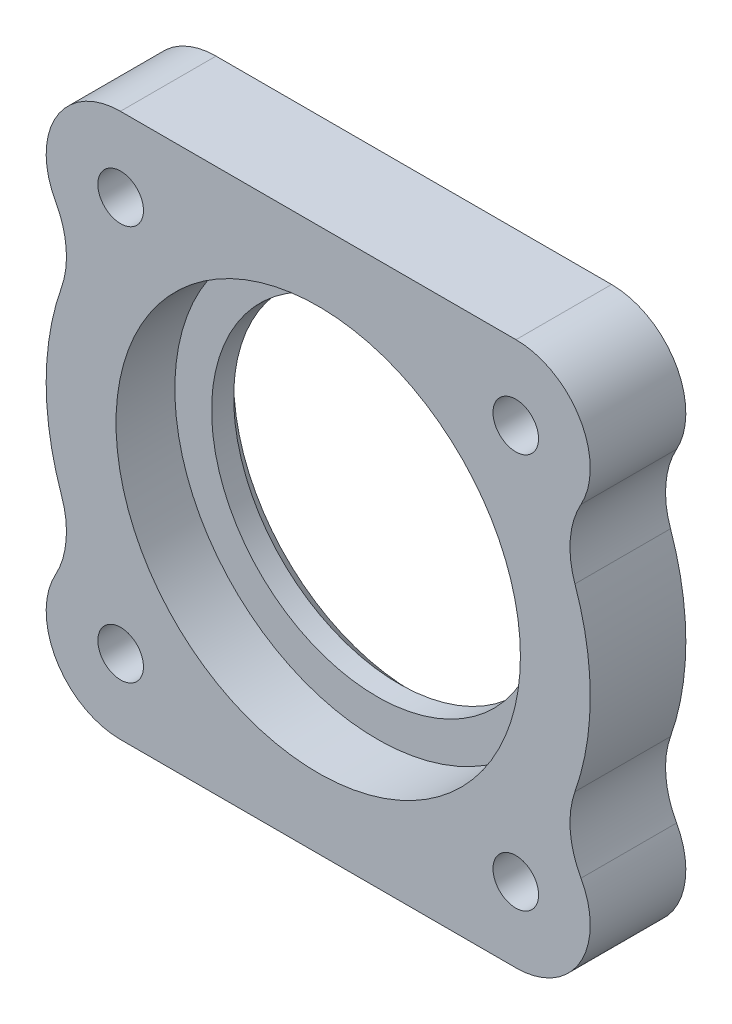
from build123d import *

# Parameters (mm, degrees)
EXTRUDE_1_DEPTH         = 13
HOLE_WIZARD_6_2_6_2_1_D = 6.2
SKETCH_4_R              = 27.5
CUT_EXTRUDE_1_DEPTH     = 8
CUT_EXTRUDE_2_REACH     = 54.934
SKETCH_5_R              = 22.5
CHAMFER_1_SIZE          = 2


with BuildPart() as part:
    # 草图1 → 凸台-拉伸1 (new body)
    with BuildSketch(Plane.XY):
        with BuildLine():
            Line((37, 0), (-37, 0))
            ThreePointArc((-37, 0), (-36.475571993, -6.2074671), (-34.917154173, -12.238968276))
            ThreePointArc((-34.917154173, -12.238968276), (-34.283867545, -17.214225736), (-35.739390486, -22.013776935))
            ThreePointArc((-35.739390486, -22.013776935), (-35.59944978, -32.031235087), (-26.9, -37))
            Line((-26.9, -37), (26.9, -37))
            ThreePointArc((26.9, -37), (35.59944978, -32.031235087), (35.739390486, -22.013776935))
            ThreePointArc((35.739390486, -22.013776935), (34.283867545, -17.214225736), (34.917154173, -12.238968276))
            ThreePointArc((34.917154173, -12.238968276), (36.475571993, -6.2074671), (37, 0))
        make_face()
        with BuildLine():
            Line((26.9, 37), (-26.9, 37))
            ThreePointArc((-26.9, 37), (-35.59944978, 32.031235087), (-35.739390486, 22.013776935))
            ThreePointArc((-35.739390486, 22.013776935), (-34.283867545, 17.214225736), (-34.917154173, 12.238968276))
            ThreePointArc((-34.917154173, 12.238968276), (-36.475571993, 6.2074671), (-37, 0))
            Line((-37, 0), (37, 0))
            ThreePointArc((37, 0), (36.475571993, 6.2074671), (34.917154173, 12.238968276))
            ThreePointArc((34.917154173, 12.238968276), (34.283867545, 17.214225736), (35.739390486, 22.013776935))
            ThreePointArc((35.739390486, 22.013776935), (35.59944978, 32.031235087), (26.9, 37))
        make_face()
    extrude(amount=EXTRUDE_1_DEPTH)

    # Ø6.2 (6.2) 直径孔1 (through all)
    with Locations(Plane(origin=(-26.870057685, 26.870057685, 13), x_dir=(1, 0, 0), z_dir=(0, 0, 1))):
        with Locations((0, 0), (53.74011537, 0), (53.74011537, -53.74011537), (0, -53.74011537)):
            Hole(HOLE_WIZARD_6_2_6_2_1_D / 2)

    # 草图4 → 切除-拉伸1 (cut)
    with BuildSketch(Plane.XY.offset(13)):
        Circle(SKETCH_4_R)
    extrude(amount=-CUT_EXTRUDE_1_DEPTH, mode=Mode.SUBTRACT)

    # 草图5 → 切除-拉伸2 (cut, up to next)
    with BuildSketch(Plane.XY.offset(5), mode=Mode.PRIVATE) as cut_extrude_2_sk1:
        Circle(SKETCH_5_R)
    cut_extrude_2_tool1 = extrude(cut_extrude_2_sk1.sketch, amount=-CUT_EXTRUDE_2_REACH, mode=Mode.PRIVATE) & part.part
    add(cut_extrude_2_tool1.solids().sort_by_distance((0, 0, 5))[0], mode=Mode.SUBTRACT)

    # 倒角1
    chamfer_1_edges = [part.edges().sort_by_distance(p)[0] for p in [
        (-22.5, 0, 0),
    ]]
    chamfer(chamfer_1_edges, length=CHAMFER_1_SIZE)


solid = part.part
